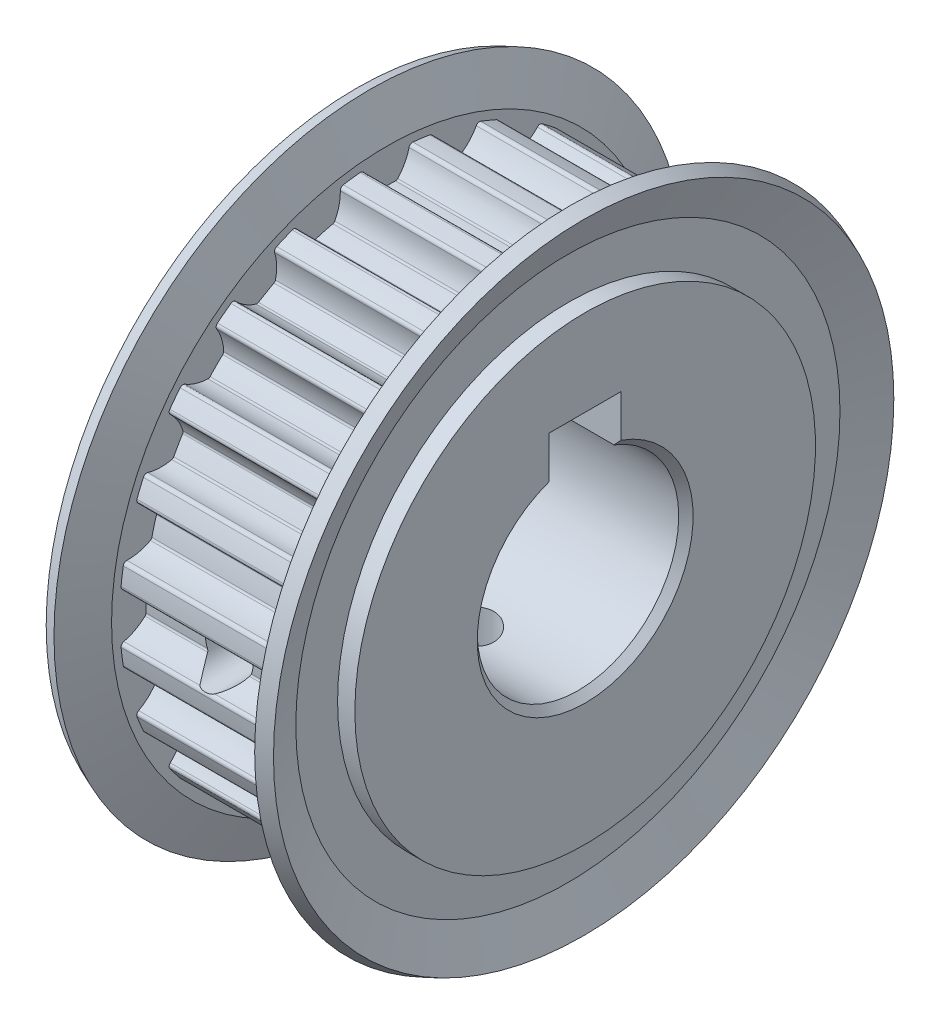
SolidWorks part; units mm, degrees
material "A7075-T6"
ref_plane "Front Plane" through (0, 0, 0) normal (0, 0, 1) x (1, 0, 0)
ref_plane "Top Plane" through (0, 0, 0) normal (0, 1, 0) x (1, 0, 0)
ref_plane "Right Plane" through (0, 0, 0) normal (1, 0, 0) x (0, 0, -1)
sketch "Sketch1" plane through (0, 0, 0) normal (0, 0, 1) x (1, 0, 0)
  line L0 (0, 16) -> (0, 4.2)
  line L1 (0, 4.2) -> (0.2, 4)
  line L2 (0.2, 4) -> (27.8, 4)
  line L3 (27.8, 4) -> (28, 4.2)
  line L4 (28, 4.2) -> (28, 12.3)
  line L5 (28, 12.3) -> (27.8, 12.5)
  line L6 (27.8, 12.5) -> (16, 12.5)
  line L7 (16, 12.5) -> (16, 16)
  line L8 (16, 16) -> (14.8, 16)
  line L9 (14.8, 16) -> (14.8, 18.9013)
  line L10 (14.8, 18.9013) -> (15.8948, 21.547)
  line L11 (15.8948, 21.547) -> (14.9708, 21.9293)
  line L12 (14.9708, 21.9293) -> (13.8, 19.1)
  line L13 (13.8, 19.1) -> (2.2, 19.1)
  line L14 (2.2, 19.1) -> (1.0292, 21.9293)
  line L15 (1.0292, 21.9293) -> (0.1052, 21.547)
  line L16 (0.1052, 21.547) -> (1.2, 18.9013)
  line L17 (1.2, 18.9013) -> (1.2, 16)
  line L18 (1.2, 16) -> (0, 16)
  line L19 (28, 0) -> (0, 0) construction
revolve "Revolve1" add sketch "Sketch1" angle 360 about L19
sketch "Sketch2" plane through (0, 0, 0) normal (0, 0, 1) x (1, 0, 0)
  line L0 (16, 0) -> (16, 13.5)
  line L1 (16, 13.5) -> (28, 13.5)
  line L2 (28, 13.5) -> (28, 0)
  line L3 (28, 0) -> (16, 0)
  line L4 (28, 0) -> (16, 0) construction
revolve "Cut-Revolve1" cut sketch "Sketch2" angle 360 about L4
ref_plane "Plane1" through (2.2, 0, 0) normal (1, 0, 0) x (0, 0, -1)
sketch "Sketch3" plane through (2.2, 0, 0) normal (1, 0, 0) x (0, 0, -1)
  line L0 (-38.2, -38.2) -> (38.2, -38.2)
  line L1 (38.2, -38.2) -> (38.2, 38.2)
  line L2 (38.2, 38.2) -> (-38.2, 38.2)
  line L3 (-38.2, 38.2) -> (-38.2, -38.2)
  arc A0 (-18.2488, -1.5673) -> (-18.4389, -1.8351) centre (-18.1901, -1.8104) ccw
  arc A1 (-18.4389, -1.8351) -> (-18.3715, -2.4187) centre (0, 0) ccw
  arc A2 (-18.3715, -2.4187) -> (-18.2856, -2.9998) centre (0, 0) ccw
  arc A3 (-18.2856, -2.9998) -> (-18.0326, -3.2092) centre (-18.0389, -2.9593) ccw
  arc A4 (-18.0326, -3.2092) -> (-16.4019, -3.5911) centre (-17.9497, -6.5282) cw
  arc A5 (-16.4019, -3.5911) -> (-16.3001, -3.7235) centre (-16.4951, -3.768) cw
  arc A6 (-16.3001, -3.7235) -> (-15.9781, -4.9254) centre (0, 0) ccw
  arc A7 (-15.9781, -4.9254) -> (-16, -5.091) centre (-16.1692, -4.9843) cw
  arc A8 (-16, -5.091) -> (-17.2213, -6.2371) centre (-18.809, -3.3213) cw
  arc A9 (-17.2213, -6.2371) -> (-17.3357, -6.5449) centre (-17.1018, -6.4566) ccw
  arc A10 (-17.3357, -6.5449) -> (-17.1195, -7.0911) centre (0, 0) ccw
  arc A11 (-17.1195, -7.0911) -> (-16.8861, -7.6302) centre (0, 0) ccw
  arc A12 (-16.8861, -7.6302) -> (-16.5876, -7.767) centre (-16.6583, -7.5273) ccw
  arc A13 (-16.5876, -7.767) -> (-14.9135, -7.7138) centre (-15.6485, -10.9515) cw
  arc A14 (-14.9135, -7.7138) -> (-14.781, -7.8154) centre (-14.9578, -7.9089) cw
  arc A15 (-14.781, -7.8154) -> (-14.1588, -8.893) centre (0, 0) ccw
  arc A16 (-14.1588, -8.893) -> (-14.1371, -9.0586) centre (-14.3282, -8.9994) cw
  arc A17 (-14.1371, -9.0586) -> (-15.0203, -10.4817) centre (-17.3085, -8.0763) cw
  arc A18 (-15.0203, -10.4817) -> (-15.051, -10.8087) centre (-14.8479, -10.6629) ccw
  arc A19 (-15.051, -10.8087) -> (-14.7008, -11.2803) centre (0, 0) ccw
  arc A20 (-14.7008, -11.2803) -> (-14.3359, -11.7407) centre (0, 0) ccw
  arc A21 (-14.3359, -11.7407) -> (-14.0121, -11.7956) centre (-14.1425, -11.5823) ccw
  arc A22 (-14.0121, -11.7956) -> (-12.4089, -11.3109) centre (-12.2808, -14.6284) cw
  arc A23 (-12.4089, -11.3109) -> (-12.2546, -11.3747) centre (-12.4012, -11.5108) cw
  arc A24 (-12.2546, -11.3747) -> (-11.3747, -12.2546) centre (0, 0) ccw
  arc A25 (-11.3747, -12.2546) -> (-11.3109, -12.4089) centre (-11.5108, -12.4012) cw
  arc A26 (-11.3109, -12.4089) -> (-11.7956, -14.0121) centre (-14.6284, -12.2808) cw
  arc A27 (-11.7956, -14.0121) -> (-11.7407, -14.3359) centre (-11.5823, -14.1425) ccw
  arc A28 (-11.7407, -14.3359) -> (-11.2803, -14.7008) centre (0, 0) ccw
  arc A29 (-11.2803, -14.7008) -> (-10.8087, -15.051) centre (0, 0) ccw
  arc A30 (-10.8087, -15.051) -> (-10.4817, -15.0203) centre (-10.6629, -14.8479) ccw
  arc A31 (-10.4817, -15.0203) -> (-9.0586, -14.1371) centre (-8.0763, -17.3085) cw
  arc A32 (-9.0586, -14.1371) -> (-8.893, -14.1588) centre (-8.9994, -14.3282) cw
  arc A33 (-8.893, -14.1588) -> (-7.8154, -14.781) centre (0, 0) ccw
  arc A34 (-7.8154, -14.781) -> (-7.7138, -14.9135) centre (-7.9089, -14.9578) cw
  arc A35 (-7.7138, -14.9135) -> (-7.767, -16.5876) centre (-10.9515, -15.6485) cw
  arc A36 (-7.767, -16.5876) -> (-7.6302, -16.8861) centre (-7.5273, -16.6583) ccw
  arc A37 (-7.6302, -16.8861) -> (-7.0911, -17.1195) centre (0, 0) ccw
  arc A38 (-7.0911, -17.1195) -> (-6.5449, -17.3357) centre (0, 0) ccw
  arc A39 (-6.5449, -17.3357) -> (-6.2371, -17.2213) centre (-6.4566, -17.1018) ccw
  arc A40 (-6.2371, -17.2213) -> (-5.091, -16) centre (-3.3213, -18.809) cw
  arc A41 (-5.091, -16) -> (-4.9254, -15.9781) centre (-4.9843, -16.1692) cw
  arc A42 (-4.9254, -15.9781) -> (-3.7235, -16.3001) centre (0, 0) ccw
  arc A43 (-3.7235, -16.3001) -> (-3.5911, -16.4019) centre (-3.768, -16.4951) cw
  arc A44 (-3.5911, -16.4019) -> (-3.2092, -18.0326) centre (-6.5282, -17.9497) cw
  arc A45 (-3.2092, -18.0326) -> (-2.9998, -18.2856) centre (-2.9593, -18.0389) ccw
  arc A46 (-2.9998, -18.2856) -> (-2.4187, -18.3715) centre (0, 0) ccw
  arc A47 (-2.4187, -18.3715) -> (-1.8351, -18.4389) centre (0, 0) ccw
  arc A48 (-1.8351, -18.4389) -> (-1.5673, -18.2488) centre (-1.8104, -18.1901) ccw
  arc A49 (-1.5673, -18.2488) -> (-0.7764, -16.7724) centre (1.66, -19.0277) cw
  arc A50 (-0.7764, -16.7724) -> (-0.6222, -16.7084) centre (-0.6296, -16.9083) cw
  arc A51 (-0.6222, -16.7084) -> (0.6222, -16.7084) centre (0, 0) ccw
  arc A52 (0.6222, -16.7084) -> (0.7764, -16.7724) centre (0.6296, -16.9083) cw
  arc A53 (0.7764, -16.7724) -> (1.5673, -18.2488) centre (-1.66, -19.0277) cw
  arc A54 (1.5673, -18.2488) -> (1.8351, -18.4389) centre (1.8104, -18.1901) ccw
  arc A55 (1.8351, -18.4389) -> (2.4187, -18.3715) centre (0, 0) ccw
  arc A56 (2.4187, -18.3715) -> (2.9998, -18.2856) centre (0, 0) ccw
  arc A57 (2.9998, -18.2856) -> (3.2092, -18.0326) centre (2.9593, -18.0389) ccw
  arc A58 (3.2092, -18.0326) -> (3.5911, -16.4019) centre (6.5282, -17.9497) cw
  arc A59 (3.5911, -16.4019) -> (3.7235, -16.3001) centre (3.768, -16.4951) cw
  arc A60 (3.7235, -16.3001) -> (4.9254, -15.9781) centre (0, 0) ccw
  arc A61 (4.9254, -15.9781) -> (5.091, -16) centre (4.9843, -16.1692) cw
  arc A62 (5.091, -16) -> (6.2371, -17.2213) centre (3.3213, -18.809) cw
  arc A63 (6.2371, -17.2213) -> (6.5449, -17.3357) centre (6.4566, -17.1018) ccw
  arc A64 (6.5449, -17.3357) -> (7.0911, -17.1195) centre (0, 0) ccw
  arc A65 (7.0911, -17.1195) -> (7.6302, -16.8861) centre (0, 0) ccw
  arc A66 (7.6302, -16.8861) -> (7.767, -16.5876) centre (7.5273, -16.6583) ccw
  arc A67 (7.767, -16.5876) -> (7.7138, -14.9135) centre (10.9515, -15.6485) cw
  arc A68 (7.7138, -14.9135) -> (7.8154, -14.781) centre (7.9089, -14.9578) cw
  arc A69 (7.8154, -14.781) -> (8.893, -14.1588) centre (0, 0) ccw
  arc A70 (8.893, -14.1588) -> (9.0586, -14.1371) centre (8.9994, -14.3282) cw
  arc A71 (9.0586, -14.1371) -> (10.4817, -15.0203) centre (8.0763, -17.3085) cw
  arc A72 (10.4817, -15.0203) -> (10.8087, -15.051) centre (10.6629, -14.8479) ccw
  arc A73 (10.8087, -15.051) -> (11.2803, -14.7008) centre (0, 0) ccw
  arc A74 (11.2803, -14.7008) -> (11.7407, -14.3359) centre (0, 0) ccw
  arc A75 (11.7407, -14.3359) -> (11.7956, -14.0121) centre (11.5823, -14.1425) ccw
  arc A76 (11.7956, -14.0121) -> (11.3109, -12.4089) centre (14.6284, -12.2808) cw
  arc A77 (11.3109, -12.4089) -> (11.3747, -12.2546) centre (11.5108, -12.4012) cw
  arc A78 (11.3747, -12.2546) -> (12.2546, -11.3747) centre (0, 0) ccw
  arc A79 (12.2546, -11.3747) -> (12.4089, -11.3109) centre (12.4012, -11.5108) cw
  arc A80 (12.4089, -11.3109) -> (14.0121, -11.7956) centre (12.2808, -14.6284) cw
  arc A81 (14.0121, -11.7956) -> (14.3359, -11.7407) centre (14.1425, -11.5823) ccw
  arc A82 (14.3359, -11.7407) -> (14.7008, -11.2803) centre (0, 0) ccw
  arc A83 (14.7008, -11.2803) -> (15.051, -10.8087) centre (0, 0) ccw
  arc A84 (15.051, -10.8087) -> (15.0203, -10.4817) centre (14.8479, -10.6629) ccw
  arc A85 (15.0203, -10.4817) -> (14.1371, -9.0586) centre (17.3085, -8.0763) cw
  arc A86 (14.1371, -9.0586) -> (14.1588, -8.893) centre (14.3282, -8.9994) cw
  arc A87 (14.1588, -8.893) -> (14.781, -7.8154) centre (0, 0) ccw
  arc A88 (14.781, -7.8154) -> (14.9135, -7.7138) centre (14.9578, -7.9089) cw
  arc A89 (14.9135, -7.7138) -> (16.5876, -7.767) centre (15.6485, -10.9515) cw
  arc A90 (16.5876, -7.767) -> (16.8861, -7.6302) centre (16.6583, -7.5273) ccw
  arc A91 (16.8861, -7.6302) -> (17.1195, -7.0911) centre (0, 0) ccw
  arc A92 (17.1195, -7.0911) -> (17.3357, -6.5449) centre (0, 0) ccw
  arc A93 (17.3357, -6.5449) -> (17.2213, -6.2371) centre (17.1018, -6.4566) ccw
  arc A94 (17.2213, -6.2371) -> (16, -5.091) centre (18.809, -3.3213) cw
  arc A95 (16, -5.091) -> (15.9781, -4.9254) centre (16.1692, -4.9843) cw
  arc A96 (15.9781, -4.9254) -> (16.3001, -3.7235) centre (0, 0) ccw
  arc A97 (16.3001, -3.7235) -> (16.4019, -3.5911) centre (16.4951, -3.768) cw
  arc A98 (16.4019, -3.5911) -> (18.0326, -3.2092) centre (17.9497, -6.5282) cw
  arc A99 (18.0326, -3.2092) -> (18.2856, -2.9998) centre (18.0389, -2.9593) ccw
  arc A100 (18.2856, -2.9998) -> (18.3715, -2.4187) centre (0, 0) ccw
  arc A101 (18.3715, -2.4187) -> (18.4389, -1.8351) centre (0, 0) ccw
  arc A102 (18.4389, -1.8351) -> (18.2488, -1.5673) centre (18.1901, -1.8104) ccw
  arc A103 (18.2488, -1.5673) -> (16.7724, -0.7764) centre (19.0277, 1.66) cw
  arc A104 (16.7724, -0.7764) -> (16.7084, -0.6222) centre (16.9083, -0.6296) cw
  arc A105 (16.7084, -0.6222) -> (16.7084, 0.6222) centre (0, 0) ccw
  arc A106 (16.7084, 0.6222) -> (16.7724, 0.7764) centre (16.9083, 0.6296) cw
  arc A107 (16.7724, 0.7764) -> (18.2488, 1.5673) centre (19.0277, -1.66) cw
  arc A108 (18.2488, 1.5673) -> (18.4389, 1.8351) centre (18.1901, 1.8104) ccw
  arc A109 (18.4389, 1.8351) -> (18.3715, 2.4187) centre (0, 0) ccw
  arc A110 (18.3715, 2.4187) -> (18.2856, 2.9998) centre (0, 0) ccw
  arc A111 (18.2856, 2.9998) -> (18.0326, 3.2092) centre (18.0389, 2.9593) ccw
  arc A112 (18.0326, 3.2092) -> (16.4019, 3.5911) centre (17.9497, 6.5282) cw
  arc A113 (16.4019, 3.5911) -> (16.3001, 3.7235) centre (16.4951, 3.768) cw
  arc A114 (16.3001, 3.7235) -> (15.9781, 4.9254) centre (0, 0) ccw
  arc A115 (15.9781, 4.9254) -> (16, 5.091) centre (16.1692, 4.9843) cw
  arc A116 (16, 5.091) -> (17.2213, 6.2371) centre (18.809, 3.3213) cw
  arc A117 (17.2213, 6.2371) -> (17.3357, 6.5449) centre (17.1018, 6.4566) ccw
  arc A118 (17.3357, 6.5449) -> (17.1195, 7.0911) centre (0, 0) ccw
  arc A119 (17.1195, 7.0911) -> (16.8861, 7.6302) centre (0, 0) ccw
  arc A120 (16.8861, 7.6302) -> (16.5876, 7.767) centre (16.6583, 7.5273) ccw
  arc A121 (16.5876, 7.767) -> (14.9135, 7.7138) centre (15.6485, 10.9515) cw
  arc A122 (14.9135, 7.7138) -> (14.781, 7.8154) centre (14.9578, 7.9089) cw
  arc A123 (14.781, 7.8154) -> (14.1588, 8.893) centre (0, 0) ccw
  arc A124 (14.1588, 8.893) -> (14.1371, 9.0586) centre (14.3282, 8.9994) cw
  arc A125 (14.1371, 9.0586) -> (15.0203, 10.4817) centre (17.3085, 8.0763) cw
  arc A126 (15.0203, 10.4817) -> (15.051, 10.8087) centre (14.8479, 10.6629) ccw
  arc A127 (15.051, 10.8087) -> (14.7008, 11.2803) centre (0, 0) ccw
  arc A128 (14.7008, 11.2803) -> (14.3359, 11.7407) centre (0, 0) ccw
  arc A129 (14.3359, 11.7407) -> (14.0121, 11.7956) centre (14.1425, 11.5823) ccw
  arc A130 (14.0121, 11.7956) -> (12.4089, 11.3109) centre (12.2808, 14.6284) cw
  arc A131 (12.4089, 11.3109) -> (12.2546, 11.3747) centre (12.4012, 11.5108) cw
  arc A132 (12.2546, 11.3747) -> (11.3747, 12.2546) centre (0, 0) ccw
  arc A133 (11.3747, 12.2546) -> (11.3109, 12.4089) centre (11.5108, 12.4012) cw
  arc A134 (11.3109, 12.4089) -> (11.7956, 14.0121) centre (14.6284, 12.2808) cw
  arc A135 (11.7956, 14.0121) -> (11.7407, 14.3359) centre (11.5823, 14.1425) ccw
  arc A136 (11.7407, 14.3359) -> (11.2803, 14.7008) centre (0, 0) ccw
  arc A137 (11.2803, 14.7008) -> (10.8087, 15.051) centre (0, 0) ccw
  arc A138 (10.8087, 15.051) -> (10.4817, 15.0203) centre (10.6629, 14.8479) ccw
  arc A139 (10.4817, 15.0203) -> (9.0586, 14.1371) centre (8.0763, 17.3085) cw
  arc A140 (9.0586, 14.1371) -> (8.893, 14.1588) centre (8.9994, 14.3282) cw
  arc A141 (8.893, 14.1588) -> (7.8154, 14.781) centre (0, 0) ccw
  arc A142 (7.8154, 14.781) -> (7.7138, 14.9135) centre (7.9089, 14.9578) cw
  arc A143 (7.7138, 14.9135) -> (7.767, 16.5876) centre (10.9515, 15.6485) cw
  arc A144 (7.767, 16.5876) -> (7.6302, 16.8861) centre (7.5273, 16.6583) ccw
  arc A145 (7.6302, 16.8861) -> (7.0911, 17.1195) centre (0, 0) ccw
  arc A146 (7.0911, 17.1195) -> (6.5449, 17.3357) centre (0, 0) ccw
  arc A147 (6.5449, 17.3357) -> (6.2371, 17.2213) centre (6.4566, 17.1018) ccw
  arc A148 (6.2371, 17.2213) -> (5.091, 16) centre (3.3213, 18.809) cw
  arc A149 (5.091, 16) -> (4.9254, 15.9781) centre (4.9843, 16.1692) cw
  arc A150 (4.9254, 15.9781) -> (3.7235, 16.3001) centre (0, 0) ccw
  arc A151 (3.7235, 16.3001) -> (3.5911, 16.4019) centre (3.768, 16.4951) cw
  arc A152 (3.5911, 16.4019) -> (3.2092, 18.0326) centre (6.5282, 17.9497) cw
  arc A153 (3.2092, 18.0326) -> (2.9998, 18.2856) centre (2.9593, 18.0389) ccw
  arc A154 (2.9998, 18.2856) -> (2.4187, 18.3715) centre (0, 0) ccw
  arc A155 (2.4187, 18.3715) -> (1.8351, 18.4389) centre (0, 0) ccw
  arc A156 (1.8351, 18.4389) -> (1.5673, 18.2488) centre (1.8104, 18.1901) ccw
  arc A157 (1.5673, 18.2488) -> (0.7764, 16.7724) centre (-1.66, 19.0277) cw
  arc A158 (0.7764, 16.7724) -> (0.6222, 16.7084) centre (0.6296, 16.9083) cw
  arc A159 (0.6222, 16.7084) -> (-0.6222, 16.7084) centre (0, 0) ccw
  arc A160 (-0.6222, 16.7084) -> (-0.7764, 16.7724) centre (-0.6296, 16.9083) cw
  arc A161 (-0.7764, 16.7724) -> (-1.5673, 18.2488) centre (1.66, 19.0277) cw
  arc A162 (-1.5673, 18.2488) -> (-1.8351, 18.4389) centre (-1.8104, 18.1901) ccw
  arc A163 (-1.8351, 18.4389) -> (-2.4187, 18.3715) centre (0, 0) ccw
  arc A164 (-2.4187, 18.3715) -> (-2.9998, 18.2856) centre (0, 0) ccw
  arc A165 (-2.9998, 18.2856) -> (-3.2092, 18.0326) centre (-2.9593, 18.0389) ccw
  arc A166 (-3.2092, 18.0326) -> (-3.5911, 16.4019) centre (-6.5282, 17.9497) cw
  arc A167 (-3.5911, 16.4019) -> (-3.7235, 16.3001) centre (-3.768, 16.4951) cw
  arc A168 (-3.7235, 16.3001) -> (-4.9254, 15.9781) centre (0, 0) ccw
  arc A169 (-4.9254, 15.9781) -> (-5.091, 16) centre (-4.9843, 16.1692) cw
  arc A170 (-5.091, 16) -> (-6.2371, 17.2213) centre (-3.3213, 18.809) cw
  arc A171 (-6.2371, 17.2213) -> (-6.5449, 17.3357) centre (-6.4566, 17.1018) ccw
  arc A172 (-6.5449, 17.3357) -> (-7.0911, 17.1195) centre (0, 0) ccw
  arc A173 (-7.0911, 17.1195) -> (-7.6302, 16.8861) centre (0, 0) ccw
  arc A174 (-7.6302, 16.8861) -> (-7.767, 16.5876) centre (-7.5273, 16.6583) ccw
  arc A175 (-7.767, 16.5876) -> (-7.7138, 14.9135) centre (-10.9515, 15.6485) cw
  arc A176 (-7.7138, 14.9135) -> (-7.8154, 14.781) centre (-7.9089, 14.9578) cw
  arc A177 (-7.8154, 14.781) -> (-8.893, 14.1588) centre (0, 0) ccw
  arc A178 (-8.893, 14.1588) -> (-9.0586, 14.1371) centre (-8.9994, 14.3282) cw
  arc A179 (-9.0586, 14.1371) -> (-10.4817, 15.0203) centre (-8.0763, 17.3085) cw
  arc A180 (-10.4817, 15.0203) -> (-10.8087, 15.051) centre (-10.6629, 14.8479) ccw
  arc A181 (-10.8087, 15.051) -> (-11.2803, 14.7008) centre (0, 0) ccw
  arc A182 (-11.2803, 14.7008) -> (-11.7407, 14.3359) centre (0, 0) ccw
  arc A183 (-11.7407, 14.3359) -> (-11.7956, 14.0121) centre (-11.5823, 14.1425) ccw
  arc A184 (-11.7956, 14.0121) -> (-11.3109, 12.4089) centre (-14.6284, 12.2808) cw
  arc A185 (-11.3109, 12.4089) -> (-11.3747, 12.2546) centre (-11.5108, 12.4012) cw
  arc A186 (-11.3747, 12.2546) -> (-12.2546, 11.3747) centre (0, 0) ccw
  arc A187 (-12.2546, 11.3747) -> (-12.4089, 11.3109) centre (-12.4012, 11.5108) cw
  arc A188 (-12.4089, 11.3109) -> (-14.0121, 11.7956) centre (-12.2808, 14.6284) cw
  arc A189 (-14.0121, 11.7956) -> (-14.3359, 11.7407) centre (-14.1425, 11.5823) ccw
  arc A190 (-14.3359, 11.7407) -> (-14.7008, 11.2803) centre (0, 0) ccw
  arc A191 (-14.7008, 11.2803) -> (-15.051, 10.8087) centre (0, 0) ccw
  arc A192 (-15.051, 10.8087) -> (-15.0203, 10.4817) centre (-14.8479, 10.6629) ccw
  arc A193 (-15.0203, 10.4817) -> (-14.1371, 9.0586) centre (-17.3085, 8.0763) cw
  arc A194 (-14.1371, 9.0586) -> (-14.1588, 8.893) centre (-14.3282, 8.9994) cw
  arc A195 (-14.1588, 8.893) -> (-14.781, 7.8154) centre (0, 0) ccw
  arc A196 (-14.781, 7.8154) -> (-14.9135, 7.7138) centre (-14.9578, 7.9089) cw
  arc A197 (-14.9135, 7.7138) -> (-16.5876, 7.767) centre (-15.6485, 10.9515) cw
  arc A198 (-16.5876, 7.767) -> (-16.8861, 7.6302) centre (-16.6583, 7.5273) ccw
  arc A199 (-16.8861, 7.6302) -> (-17.1195, 7.0911) centre (0, 0) ccw
  arc A200 (-17.1195, 7.0911) -> (-17.3357, 6.5449) centre (0, 0) ccw
  arc A201 (-17.3357, 6.5449) -> (-17.2213, 6.2371) centre (-17.1018, 6.4566) ccw
  arc A202 (-17.2213, 6.2371) -> (-16, 5.091) centre (-18.809, 3.3213) cw
  arc A203 (-16, 5.091) -> (-15.9781, 4.9254) centre (-16.1692, 4.9843) cw
  arc A204 (-15.9781, 4.9254) -> (-16.3001, 3.7235) centre (0, 0) ccw
  arc A205 (-16.3001, 3.7235) -> (-16.4019, 3.5911) centre (-16.4951, 3.768) cw
  arc A206 (-16.4019, 3.5911) -> (-18.0326, 3.2092) centre (-17.9497, 6.5282) cw
  arc A207 (-18.0326, 3.2092) -> (-18.2856, 2.9998) centre (-18.0389, 2.9593) ccw
  arc A208 (-18.2856, 2.9998) -> (-18.3715, 2.4187) centre (0, 0) ccw
  arc A209 (-18.3715, 2.4187) -> (-18.4389, 1.8351) centre (0, 0) ccw
  arc A210 (-18.4389, 1.8351) -> (-18.2488, 1.5673) centre (-18.1901, 1.8104) ccw
  arc A211 (-18.2488, 1.5673) -> (-16.7724, 0.7764) centre (-19.0277, -1.66) cw
  arc A212 (-16.7724, 0.7764) -> (-16.7084, 0.6222) centre (-16.9083, 0.6296) cw
  arc A213 (-16.7084, 0.6222) -> (-16.7084, -0.6222) centre (0, 0) ccw
  arc A214 (-16.7084, -0.6222) -> (-16.7724, -0.7764) centre (-16.9083, -0.6296) cw
  arc A215 (-16.7724, -0.7764) -> (-18.2488, -1.5673) centre (-19.0277, 1.66) cw
extrude "Cut-Extrude1" cut sketch "Sketch3" along normal blind 11.6
ref_plane "Plane2" through (8, 0, 0) normal (1, 0, 0) x (0, 0, -1)
sketch "Sketch4" plane through (16, 0, 0) normal (1, 0, 0) x (0, 0, -1)
  circle A0 centre (0, 0) radius 7
  dimension "D1" = 14
extrude "Cut-Extrude2" cut sketch "Sketch4" against normal through all
sketch "Sketch7" plane through (0, 0, 0) normal (0, 0, 1) x (1, 0, 0)
  line L1 (-5.6429, 10) -> (19.4773, 10)
  line L2 (-5.6429, 10) -> (-5.6429, 1.9995)
  line L3 (-5.6429, 1.9995) -> (19.4773, 1.9995)
  line L4 (19.4773, 10) -> (19.4773, 1.9995)
  dimension "D2" = 10
extrude "Cut-Extrude3" cut sketch "Sketch7" against normal mid plane 5
hole_wizard "M4 Tapped Hole1" positions "Sketch10" profile "Sketch9" tap size "M4" standard "Gb"
sketch "Sketch10" plane through (0, 0, 0) normal (0, 1, 0) x (1, 0, 0)
  line L1 (8, 18.4389) -> (8, -20.9254) construction
  line L2 (13.8, 18.4389) -> (2.2, 18.4389) construction
  point P0 (8, 0)
sketch "Sketch9" plane through (8, 0, 0) normal (1, 0, 0) x (0, 0, 1)
  line L0 (0, 0) -> (0, 21.9293)
  line L1 (0, 21.9293) -> (1.65, 21.9293)
  line L2 (1.65, 21.9293) -> (1.65, 0)
  line L5 (1.65, 0) -> (0, 0)
  line L11 (0, -6.35) -> (0, 107.95) construction
  dimension "通孔螺纹孔钻头直径" = 3.3
  dimension "通孔螺纹孔钻头深度" = 21.9293
cosmetic thread "Cosmetic Thread1" parameters "D2"=4
hole_wizard "M4 Tapped Hole2" positions "Sketch12" profile "Sketch11" tap size "M4" standard "Gb"
sketch "Sketch12" plane through (0, 0, 0) normal (0, 0, 1) x (1, 0, 0)
  line L0 (8, 18.2856) -> (8, -22.9136) construction
  line L1 (13.8, 18.2856) -> (2.2, 18.2856) construction
  point P0 (8, 0)
cosmetic thread "Cosmetic Thread2" parameters "D2"=4
sketch "Sketch11" plane through (8, 0, 0) normal (1, 0, 0) x (0, 1, 0)
  line L0 (0, 0) -> (0, 21.9293)
  line L1 (0, 21.9293) -> (1.65, 21.9293)
  line L2 (1.65, 21.9293) -> (1.65, 0)
  line L5 (1.65, 0) -> (0, 0)
  line L11 (0, -6.35) -> (0, 107.95) construction
  dimension "通孔螺纹孔钻头直径" = 3.3
  dimension "通孔螺纹孔钻头深度" = 21.9293
chamfer "Chamfer1" distance 0.5 angle 45 2 edges at (0, -7, 0) (16, -7, 0)
